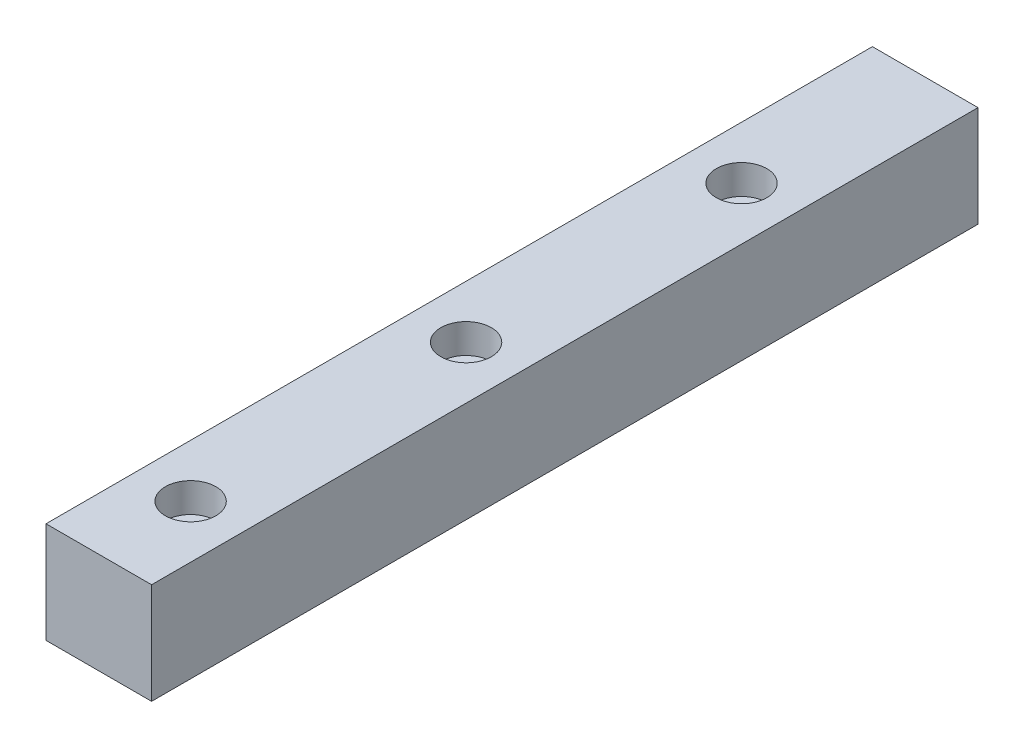
from build123d import *

# Parameters (mm, degrees)
SKETCH_1_W                   = 23
SKETCH_1_H                   = 22
EXTRUDE_1_DEPTH              = 180
HOLE_WIZARD_M6_1_D           = 6.6
HOLE_WIZARD_M6_1_CBORE_D     = 11
HOLE_WIZARD_M6_1_CBORE_DEPTH = 6.4
PATTERN_LINEAR_1_COUNT       = 4
PATTERN_LINEAR_1_PITCH       = 60


with BuildPart() as part:
    # 草图1 → 凸台-拉伸1 (new body)
    with BuildSketch(Plane.XY):
        with Locations((11.5, 11)):
            Rectangle(SKETCH_1_W, SKETCH_1_H)
    extrude(amount=EXTRUDE_1_DEPTH)

    # M6 六角凹头螺钉的柱形沉头孔1 (through all)
    with Locations(Plane(origin=(0, 22, 0), x_dir=(1, 0, 0), z_dir=(0, 1, 0))):
        with Locations((11.5, -160)):
            hole_wizard_m6_1 = CounterBoreHole(HOLE_WIZARD_M6_1_D / 2, HOLE_WIZARD_M6_1_CBORE_D / 2, HOLE_WIZARD_M6_1_CBORE_DEPTH)

    # 阵列(线性)1: M6 六角凹头螺钉的柱形沉头孔1 ×4
    with Locations(*[(0, 0, -i * PATTERN_LINEAR_1_PITCH) for i in range(1, PATTERN_LINEAR_1_COUNT)]):
        add(hole_wizard_m6_1, mode=Mode.SUBTRACT)


solid = part.part
